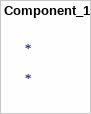
[diagram p0: symbol Component_1]
# Altium schematic symbol library MISC82375-17.SchLib: 1 symbol
Pins are listed as number, name and electrical type; pins without a type are passive.


## Component_1
designator *